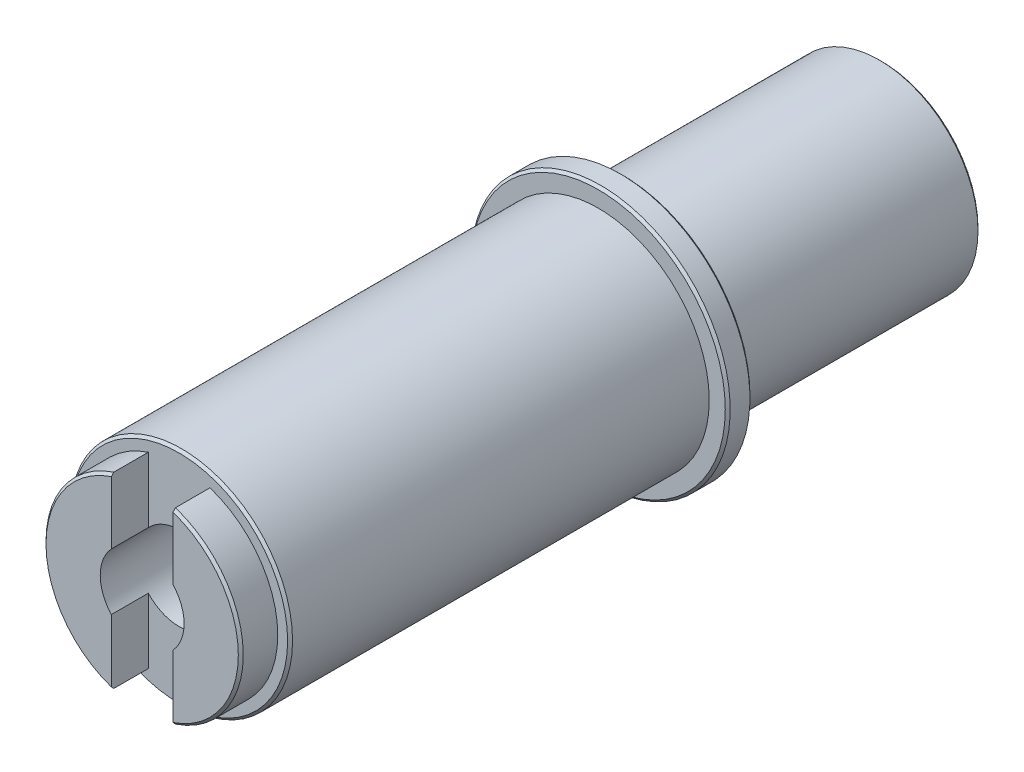
from build123d import *

# Parameters (mm, degrees)
SKETCH_1_R             = 9
EXTRUDE_1_DEPTH        = 34
SKETCH_2_R             = 8
EXTRUDE_2_DEPTH        = 3
SKETCH_3_R             = 10.5
EXTRUDE_3_DEPTH        = 2
EXTRUDE_START          = 21
SKETCH_4_R             = 8
EXTRUDE_4_DEPTH        = 21
SKETCH_5_W             = 5
SKETCH_5_H             = 32.45039325
CUT_EXTRUDE_1_DEPTH    = 3
HOLE_WIZARD_M8_1_D     = 6.8
HOLE_WIZARD_M8_1_DEPTH = 19.75
HOLE_WIZARD_M8_1_TIP   = 2.042926105
CHAMFER_1_SIZE         = 0.2


with BuildPart() as part:
    # 草图1 → 凸台-拉伸1 (new body)
    with BuildSketch(Plane.XY):
        Circle(SKETCH_1_R)
    extrude(amount=EXTRUDE_1_DEPTH)

    # 草图2 → 凸台-拉伸2 (add)
    with BuildSketch(Plane.XY.offset(34)):
        Circle(SKETCH_2_R)
    extrude(amount=EXTRUDE_2_DEPTH)

    # 草图3 → 凸台-拉伸3 (add)
    with BuildSketch(Plane(origin=(0, 0, 0), x_dir=(-1, 0, 0), z_dir=(0, 0, -1))):
        Circle(SKETCH_3_R)
    extrude(amount=EXTRUDE_3_DEPTH)

    # 草图4 → 凸台-拉伸4 (add)
    with BuildSketch(Plane(origin=(0, 0, -2), x_dir=(-1, 0, 0), z_dir=(0, 0, -1)).offset(EXTRUDE_START)):
        with Locations(Location((0, 0, 0), (0, 0, 180))):
            Circle(SKETCH_4_R)
    extrude(amount=-EXTRUDE_4_DEPTH)

    # 草图5 → 切除-拉伸1 (cut)
    with BuildSketch(Plane.XY.offset(37)):
        with Locations((0, 1.931578492)):
            Rectangle(SKETCH_5_W, SKETCH_5_H)
    extrude(amount=-CUT_EXTRUDE_1_DEPTH, mode=Mode.SUBTRACT)

    # M8 螺纹孔1
    with Locations(Plane.XY.offset(37)):
        with Locations((0, 0)):
            Hole(HOLE_WIZARD_M8_1_D / 2, depth=HOLE_WIZARD_M8_1_DEPTH)
            with Locations((0, 0, -(HOLE_WIZARD_M8_1_DEPTH + HOLE_WIZARD_M8_1_TIP / 2))):  # 118° drill point
                Cone(0, HOLE_WIZARD_M8_1_D / 2, HOLE_WIZARD_M8_1_TIP, mode=Mode.SUBTRACT)

    # 倒角1
    chamfer_1_edges = [part.edges().sort_by_distance(p)[0] for p in [
        (10.5, 0, -2),
        (-8, 0, -23),
        (-9, 0, 34),
        (-8, 0, 37),
        (8, 0, 37),
        (10.5, 0, 0),
    ]]
    chamfer(chamfer_1_edges, length=CHAMFER_1_SIZE)


solid = part.part
